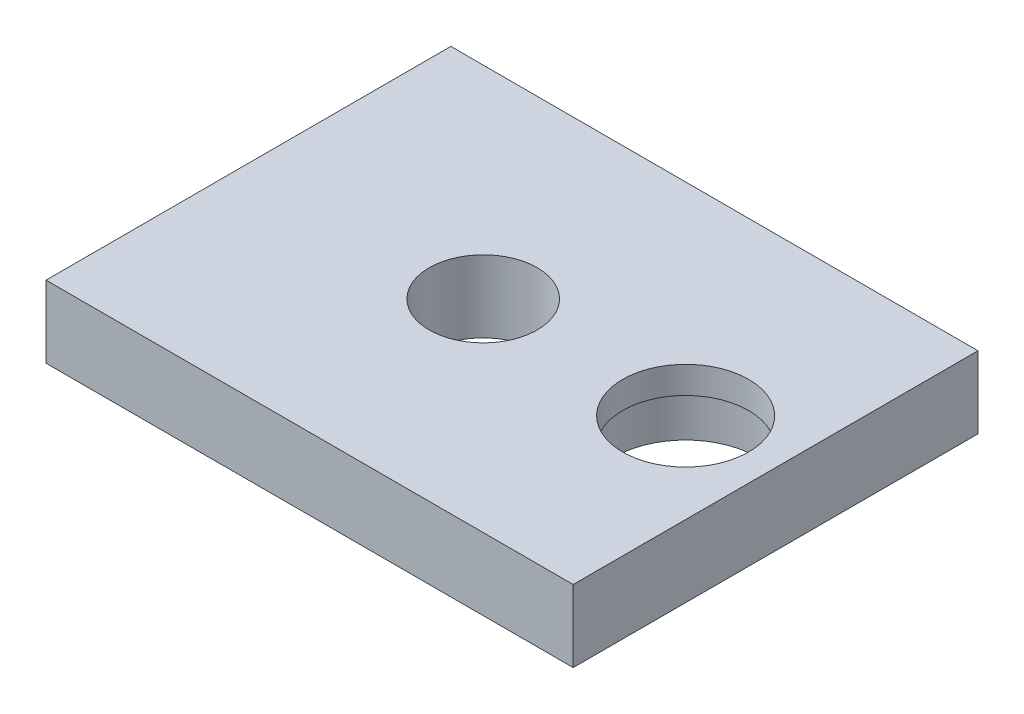
from build123d import *

# Parameters (mm, degrees)
SKETCH_1_W          = 293
SKETCH_1_H          = 225
EXTRUDE_1_DEPTH     = 40
SKETCH_2_R          = 40
CUT_EXTRUDE_1_DEPTH = 25
SKETCH_3_R          = 30
CUT_EXTRUDE_2_DEPTH = 189.993386128
SKETCH_4_R          = 35
CUT_EXTRUDE_3_DEPTH = 189.993386128


with BuildPart() as part:
    # 草图1 → 凸台-拉伸1 (new body)
    with BuildSketch(Plane(origin=(0, 0, 0), x_dir=(1, 0, 0), z_dir=(0, 1, 0))):
        Rectangle(SKETCH_1_W, SKETCH_1_H)
    extrude(amount=EXTRUDE_1_DEPTH)

    # 草图2 → 切除-拉伸1 (cut)
    with BuildSketch(Plane.XZ):
        with Locations(Location((96.5, 0, 0), (0, 0, 270))):
            Circle(SKETCH_2_R)
    extrude(amount=-CUT_EXTRUDE_1_DEPTH, mode=Mode.SUBTRACT)

    # 草图3 → 切除-拉伸2 (cut, through all)
    with BuildSketch(Plane.XZ):
        with Locations(Location((-16, 0, 0), (0, 0, 270))):
            Circle(SKETCH_3_R)
    extrude(amount=-CUT_EXTRUDE_2_DEPTH, mode=Mode.SUBTRACT)

    # 草图4 → 切除-拉伸3 (cut, through all)
    with BuildSketch(Plane.XZ):
        with Locations(Location((96.5, 0, 0), (0, 0, 270))):
            Circle(SKETCH_4_R)
    extrude(amount=-CUT_EXTRUDE_3_DEPTH, mode=Mode.SUBTRACT)


solid = part.part
